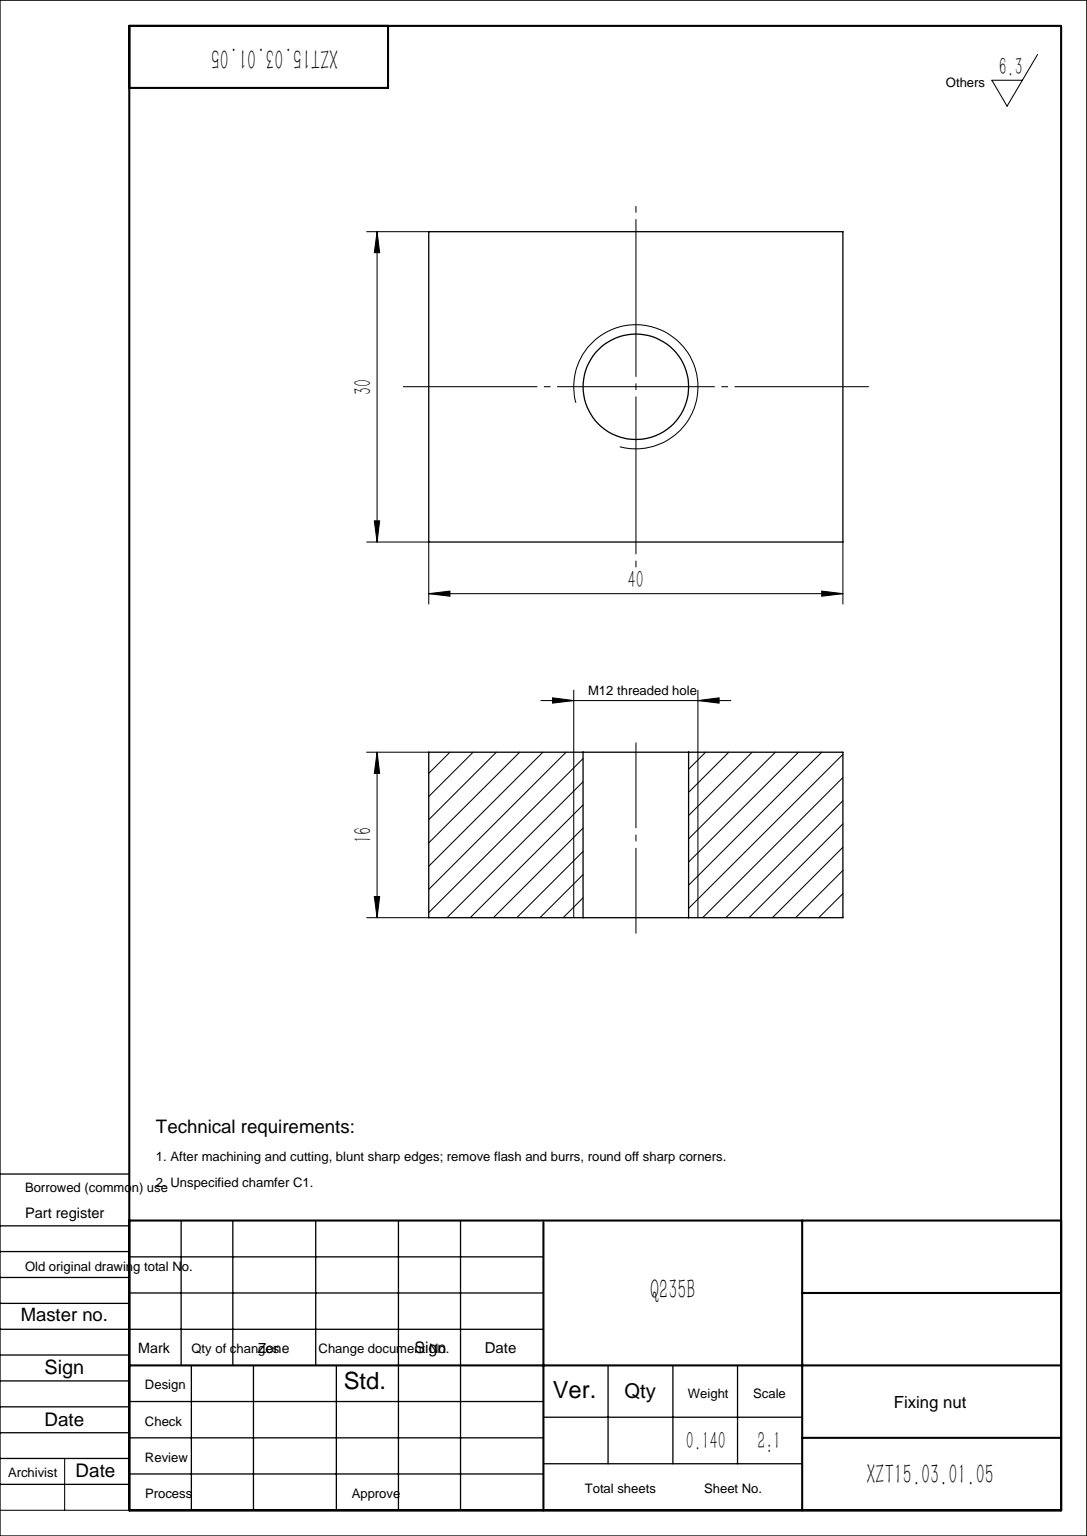
SolidWorks part; units mm, degrees
material "Q235B"
ref_plane "Front Plane" through (0, 0, 0) normal (0, 0, 1) x (1, 0, 0)
ref_plane "Top Plane" through (0, 0, 0) normal (0, 1, 0) x (1, 0, 0)
ref_plane "Right Plane" through (0, 0, 0) normal (1, 0, 0) x (0, 0, -1)
sketch "Sketch1" plane through (0, 0, 0) normal (0, 1, 0) x (1, 0, 0)
  line L1 (20, -15) -> (-20, -15)
  line L2 (20, -15) -> (20, 15)
  line L3 (20, 15) -> (-20, 15)
  line L4 (-20, -15) -> (-20, 15)
  line L5 (20, -15) -> (-20, 15) construction
  line L6 (20, 15) -> (-20, -15) construction
  point P0 (0, 0)
  dimension "D1" = 30
  dimension "D2" = 40
extrude "Boss-Extrude1" add sketch "Sketch1" along normal blind 16
hole_wizard "M12 Tapped Hole1" positions "Sketch2" profile "Sketch3" tap size "M12" standard "GB" end condition up to next
sketch "Sketch2" plane through (0, 16, 0) normal (0, 1, 0) x (1, 0, 0)
  point P0 (0, 0)
sketch "Sketch3" plane through (0, 16, 0) normal (1, 0, 0) x (0, 0, 1)
  line L0 (0, 0) -> (0, 16)
  line L1 (0, 16) -> (5.1, 16)
  line L2 (5.1, 16) -> (5.1, 0)
  line L5 (5.1, 0) -> (0, 0)
  line L11 (0, -6.35) -> (0, 107.95) construction
  dimension "通孔螺纹孔钻头直径" = 10.2
  dimension "通孔螺纹孔钻头深度" = 16
cosmetic thread "CosmeticThread Hole Thread1"
